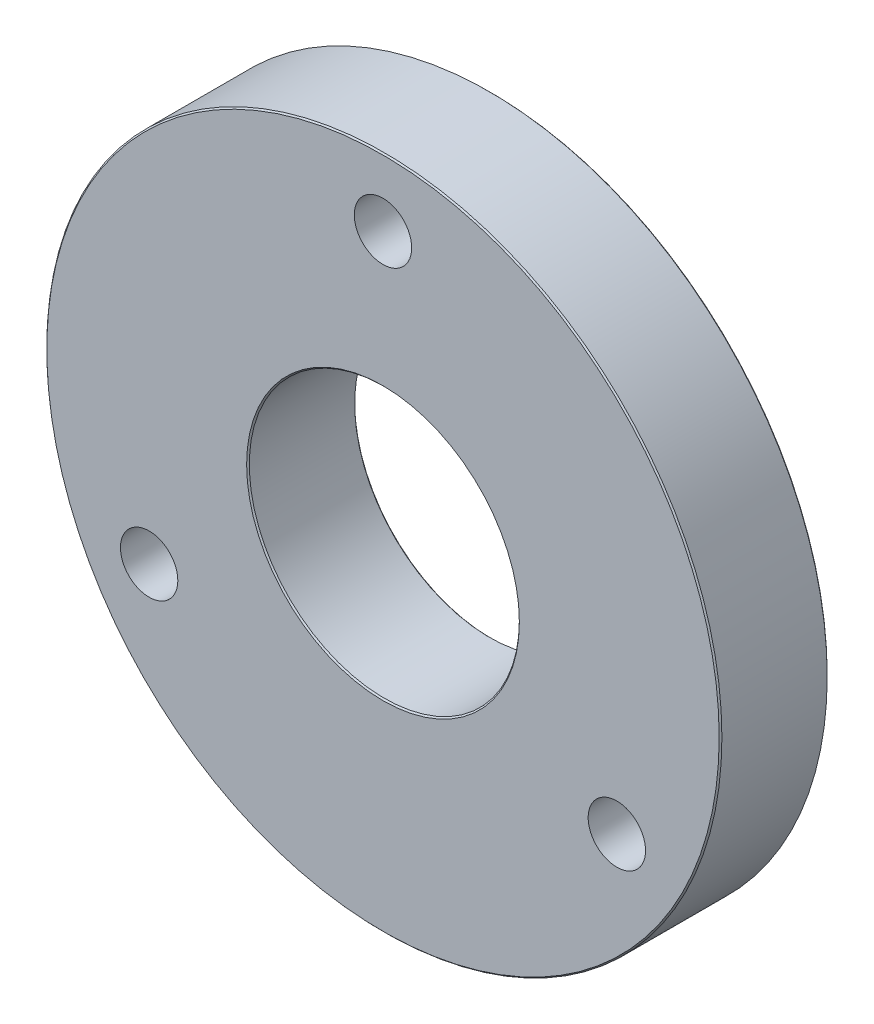
from build123d import *

# Parameters (mm, degrees)
SKETCH1_R           = 50
SKETCH1_R_2         = 20
BOSS_EXTRUDE1_DEPTH = 16
CIRPATTERN1_COUNT   = 3
CHAMFER1_SIZE       = 0.2


with BuildPart() as part:
    # Sketch1 → Boss-Extrude1 (new body)
    with BuildSketch(Plane.XY):
        Circle(SKETCH1_R)
        Circle(SKETCH1_R_2, mode=Mode.SUBTRACT)
    extrude(amount=BOSS_EXTRUDE1_DEPTH)

    # Sketch5 → M10 Tapped Hole1 (revolve, cut)
    with BuildSketch(Plane(origin=(0, 40, 16), x_dir=(0, -1, 0), z_dir=(1, 0, 0))):
        Polygon((0, 0), (0, 31.803657631), (4.25, 29.25), (4.25, 0), align=None)
    m10_tapped_hole1 = revolve(axis=Axis((0, 40, 22.35), (0, 0, -1)), mode=Mode.SUBTRACT)

    # CirPattern1: M10 Tapped Hole1 ×3 about axis
    cirpattern1_axis = Axis((0, 0, 0), (0, 0, 1))
    for i in range(1, CIRPATTERN1_COUNT):
        add(m10_tapped_hole1.rotate(cirpattern1_axis, i * 360 / CIRPATTERN1_COUNT), mode=Mode.SUBTRACT)

    # Chamfer1
    chamfer1_edges = [part.edges().sort_by_distance(p)[0] for p in [
        (-50, 0, 0),
        (-50, 0, 16),
        (-20, 0, 0),
        (-20, 0, 16),
    ]]
    chamfer(chamfer1_edges, length=CHAMFER1_SIZE)


solid = part.part
